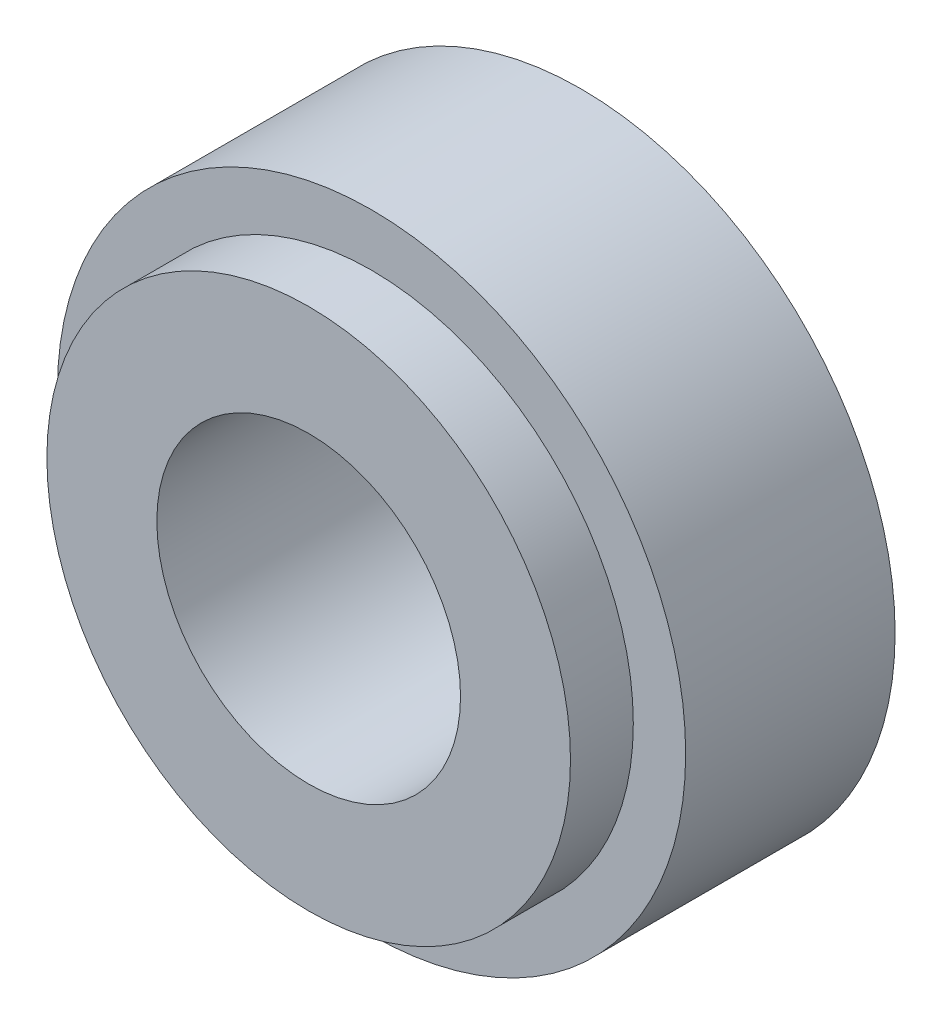
from build123d import *

# Parameters (mm, degrees)
SKETCH1_R                  = 15
BOSS_EXTRUDE1_DEPTH        = 10
SKETCH2_R                  = 12.5
BOSS_EXTRUDE2_DEPTH        = 3
SKETCH3_R                  = 6
CUT_EXTRUDE1_DEPTH         = 25.879710609
M16X1_5_TAPPED_HOLE1_D     = 14.5
M16X1_5_TAPPED_HOLE1_DEPTH = 39.5
M16X1_5_TAPPED_HOLE1_TIP   = 4.356239488


with BuildPart() as part:
    # Sketch1 → Boss-Extrude1 (new body)
    with BuildSketch(Plane.XY):
        Circle(SKETCH1_R)
    extrude(amount=BOSS_EXTRUDE1_DEPTH)

    # Sketch2 → Boss-Extrude2 (add)
    with BuildSketch(Plane.XY.offset(10)):
        Circle(SKETCH2_R)
    extrude(amount=BOSS_EXTRUDE2_DEPTH)

    # Sketch3 → Cut-Extrude1 (cut, through all)
    with BuildSketch(Plane.XY.offset(13)):
        Circle(SKETCH3_R)
    extrude(amount=-CUT_EXTRUDE1_DEPTH, mode=Mode.SUBTRACT)

    # M16x1.5 Tapped Hole1
    with Locations(Plane(origin=(0, 0, 0), x_dir=(-1, 0, 0), z_dir=(0, 0, -1))):
        with Locations((0, 0)):
            Hole(M16X1_5_TAPPED_HOLE1_D / 2, depth=M16X1_5_TAPPED_HOLE1_DEPTH)
            with Locations((0, 0, -(M16X1_5_TAPPED_HOLE1_DEPTH + M16X1_5_TAPPED_HOLE1_TIP / 2))):  # 118° drill point
                Cone(0, M16X1_5_TAPPED_HOLE1_D / 2, M16X1_5_TAPPED_HOLE1_TIP, mode=Mode.SUBTRACT)


solid = part.part
